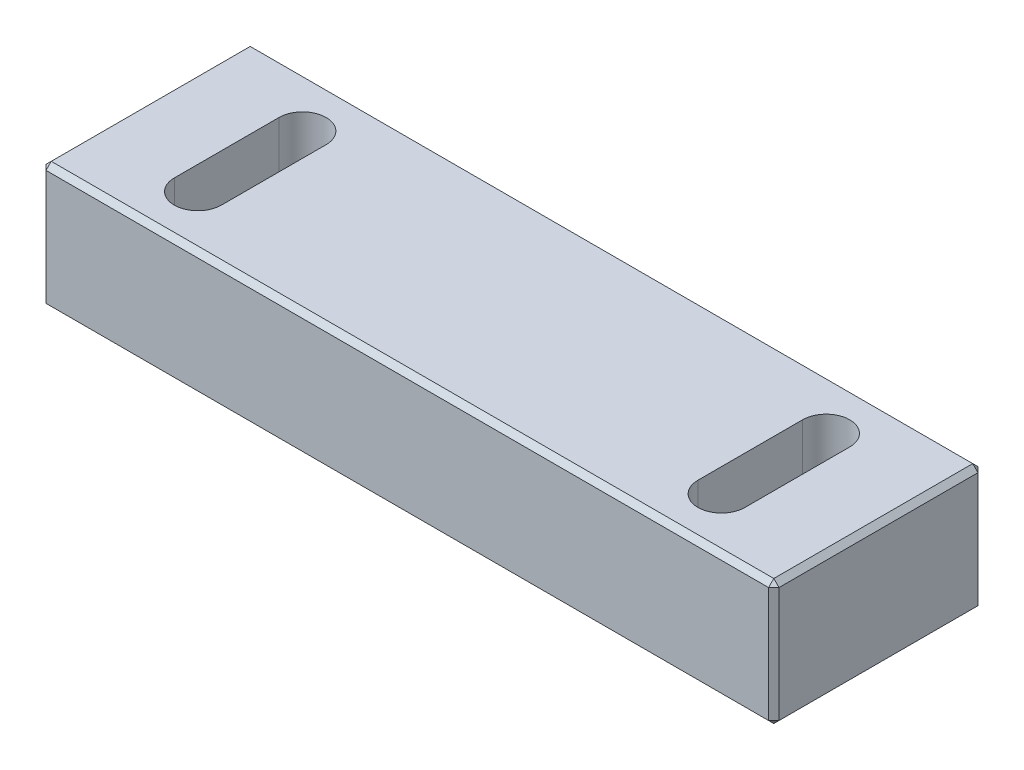
from build123d import *

# Parameters (mm, degrees)
SKETCH1_W          = 70
SKETCH1_H          = 20
EXTRUDE1_DEPTH     = 12
CUT_EXTRUDE1_DEPTH = 39.327535793
CHAMFER1_SIZE      = 0.5


with BuildPart() as part:
    # Sketch1 → Extrude1 (new body)
    with BuildSketch(Plane(origin=(0, 0, 0), x_dir=(1, 0, 0), z_dir=(0, 1, 0))):
        Rectangle(SKETCH1_W, SKETCH1_H)
    extrude(amount=EXTRUDE1_DEPTH)

    # Sketch2 → Cut-Extrude1 (cut, through all)
    with BuildSketch(Plane(origin=(0, 12, 0), x_dir=(1, 0, 0), z_dir=(0, 1, 0))):
        with BuildLine():
            Line((22.75, 5), (22.75, -5))
            ThreePointArc((22.75, -5), (25, -7.25), (27.25, -5))
            Line((27.25, -5), (27.25, 5))
            ThreePointArc((27.25, 5), (25, 7.25), (22.75, 5))
        make_face()
        with BuildLine():
            Line((-27.25, 5), (-27.25, -5))
            ThreePointArc((-27.25, -5), (-25, -7.25), (-22.75, -5))
            Line((-22.75, -5), (-22.75, 5))
            ThreePointArc((-22.75, 5), (-25, 7.25), (-27.25, 5))
        make_face()
    extrude(amount=-CUT_EXTRUDE1_DEPTH, mode=Mode.SUBTRACT)

    # Chamfer1
    chamfer1_edges = [part.edges().sort_by_distance(p)[0] for p in [
        (35, 12, 0),
        (0, 12, -10),
        (-35, 12, 0),
        (0, 0, -10),
        (35, 0, 0),
        (0, 0, 10),
        (-35, 0, 0),
        (0, 12, 10),
        (-35, 6, -10),
        (35, 6, -10),
        (35, 6, 10),
        (-35, 6, 10),
    ]]
    chamfer(chamfer1_edges, length=CHAMFER1_SIZE)


solid = part.part
